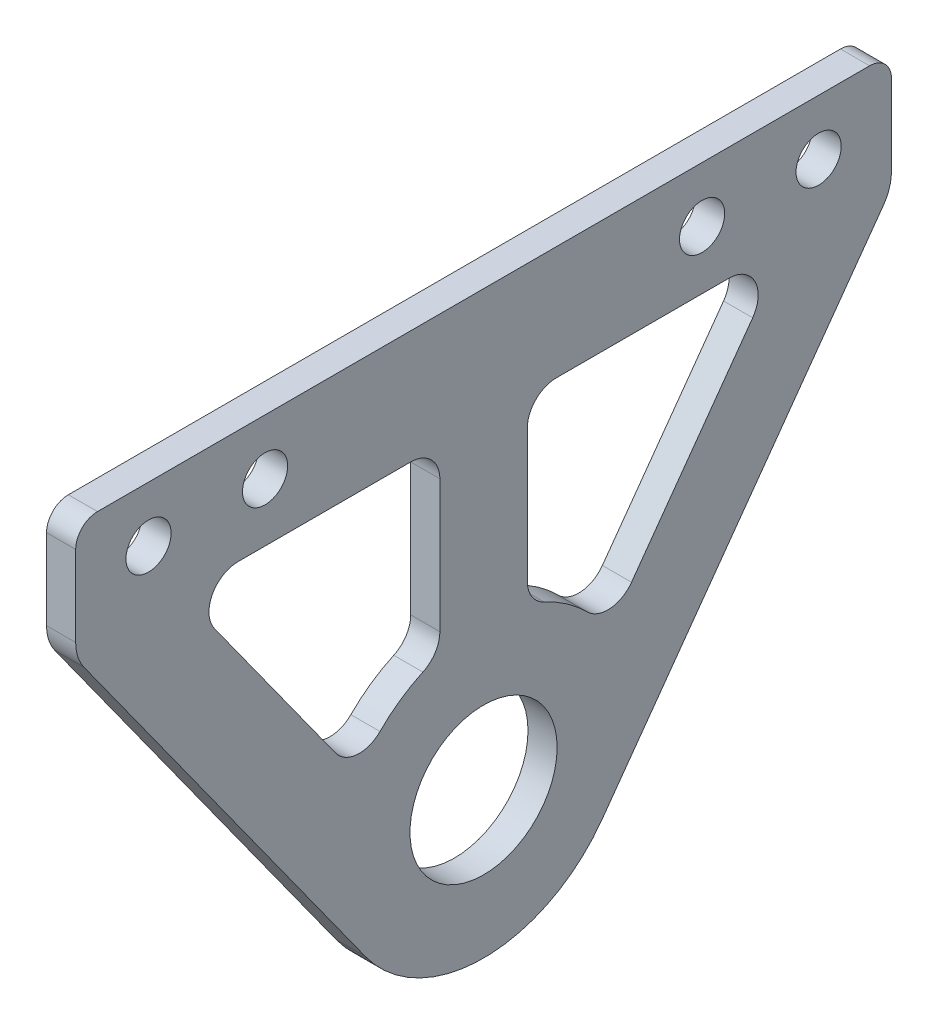
SolidWorks part; units mm, degrees
material "Thornel Mat VMA"
ref_plane "前视基准面" through (0, 0, 0) normal (0, 0, 1) x (1, 0, 0)
ref_plane "上视基准面" through (0, 0, 0) normal (0, 1, 0) x (1, 0, 0)
ref_plane "右视基准面" through (0, 0, 0) normal (1, 0, 0) x (0, 0, -1)
other "Configuration Table"
sketch "草图1" plane through (0, 0, 0) normal (1, 0, 0) x (0, 0, -1)
  line L0 (0, 0) -> (0, 29.8) construction
  line L1 (0, 29.8) -> (-15, 29.8) construction
  line L2 (-15, 29.8) -> (-15, 26) construction
  line L3 (-15, 29.8) -> (-23, 29.8) construction
  line L4 (-23, 29.8) -> (-23, 26) construction
  line L5 (-23, 29.8) -> (-28, 29.8) construction
  line L6 (-28, 29.8) -> (-28, 21.8)
  line L7 (28, 29.8) -> (-28, 29.8)
  line L8 (-28, 21.8) -> (-8.1179, -5.8395)
  line L9 (28, 29.8) -> (28, 21.8)
  line L10 (28, 21.8) -> (8.1179, -5.8395)
  circle A0 centre (0, 0) radius 5.05
  circle A1 centre (-15, 26) radius 1.55
  circle A2 centre (-23, 26) radius 1.55
  arc A3 (-8.1179, -5.8395) -> (8.1179, -5.8395) centre (0, 0) ccw
  circle A4 centre (23, 26) radius 1.55
  circle A5 centre (15, 26) radius 1.55
  dimension "D1" = 10.1
  dimension "D7" = 3.1
  dimension "D8" = 3.1
  dimension "D9" = 20
  dimension "D2" = 29.8
  dimension "D3" = 15
  dimension "D4" = 3.8
  dimension "D5" = 8
  dimension "D6" = 3.8
  dimension "D10" = 28
  dimension "D11" = 8
extrude "凸台-拉伸1" add sketch "草图1" along normal blind 2
sketch "草图2" plane through (0, 0, 0) normal (1, 0, 0) x (0, 0, -1)
  line L0 (-20.7528, 22) -> (-8.5991, 5.1044) construction
  line L1 (0, 0) -> (15, 26) construction
  line L2 (15, 26) -> (-15, 26) construction
  line L3 (0, 0) -> (0, 26) construction
  line L4 (-3, 22) -> (-3, 9.5394)
  line L5 (-28, 21.8) -> (-8.1179, -5.8395) construction
  line L6 (-20.7528, 22) -> (-8.5991, 5.1044)
  line L7 (-20.7528, 22) -> (-3, 22)
  arc A0 (-3, 9.5394) -> (-8.5991, 5.1044) centre (0, 0) ccw
  dimension "D1" = 20
  dimension "D3" = 6
  dimension "D2" = 3
  dimension "D4" = 8
extrude "切除-拉伸1" cut sketch "草图2" along normal through all
fillet "圆角1" radius 2 4 edges at (1, 22, 3) (1, 9.5394, 3) (1, 5.1044, 8.5991) (1, 22, 20.7528)
mirror "镜向1" about plane through (0, 0, 0) normal (0, 0, 1) of "切除-拉伸1"
fillet "圆角2" radius 2 4 edges at (1, 22, -20.7528) (1, 5.1044, -8.5991) (1, 9.5394, -3) (1, 22, -3)
fillet "圆角3" radius 3 2 edges at (1, 21.8, 28) (1, 21.8, -28)
fillet "圆角4" radius 1.5 2 edges at (1, 29.8, -28) (1, 29.8, 28)
